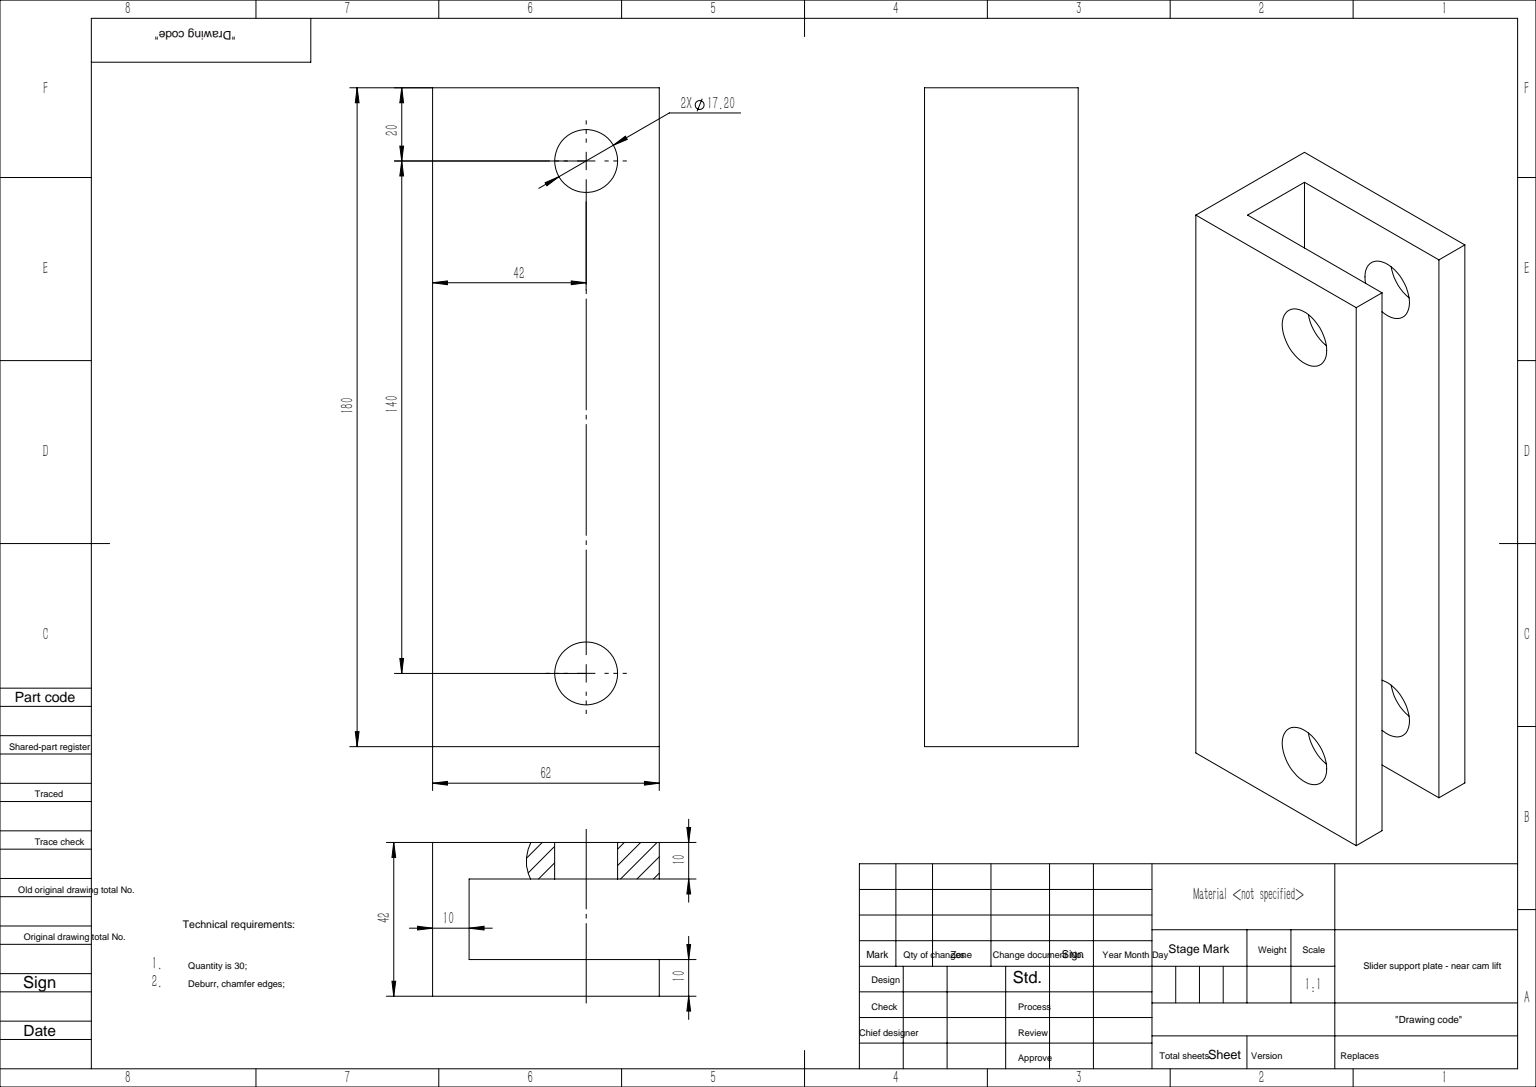
SolidWorks part; units mm, degrees
ref_plane "前视基准面" through (0, 0, 0) normal (0, 0, 1) x (1, 0, 0)
ref_plane "上视基准面" through (0, 0, 0) normal (0, 1, 0) x (1, 0, 0)
ref_plane "右视基准面" through (0, 0, 0) normal (1, 0, 0) x (0, 0, -1)
sketch "草图1" plane through (0, 0, 0) normal (0, 1, 0) x (1, 0, 0)
  line L0 (0, 0) -> (103.7045, 0) construction
  line L1 (62, 11) -> (10, 11)
  line L2 (0, 21) -> (62, 21)
  line L3 (0, 21) -> (0, -21)
  line L4 (0, -21) -> (62, -21)
  line L5 (62, 21) -> (62, 11)
  line L6 (10, 11) -> (10, -11)
  line L7 (10, -11) -> (62, -11)
  line L8 (62, -11) -> (62, -21)
  dimension "D1" = 42
  dimension "D2" = 10
  dimension "D3" = 62
  dimension "D4" = 10
extrude "凸台-拉伸1" add sketch "草图1" along normal blind 180
sketch "草图2" plane through (0, 0, 21) normal (0, 0, 1) x (1, 0, 0)
  line L0 (62, 180) -> (62, 0) construction
  line L1 (0, 180) -> (62, 180) construction
  line L2 (0, 90) -> (62, 90) construction
  line L3 (0, 180) -> (0, 0) construction
  circle A0 centre (42, 160) radius 8.6
  circle A1 centre (42, 20) radius 8.6
  dimension "D1" = 17.2
  dimension "D2" = 20
  dimension "D3" = 20
extrude "切除-拉伸1" cut sketch "草图2" against normal through all
